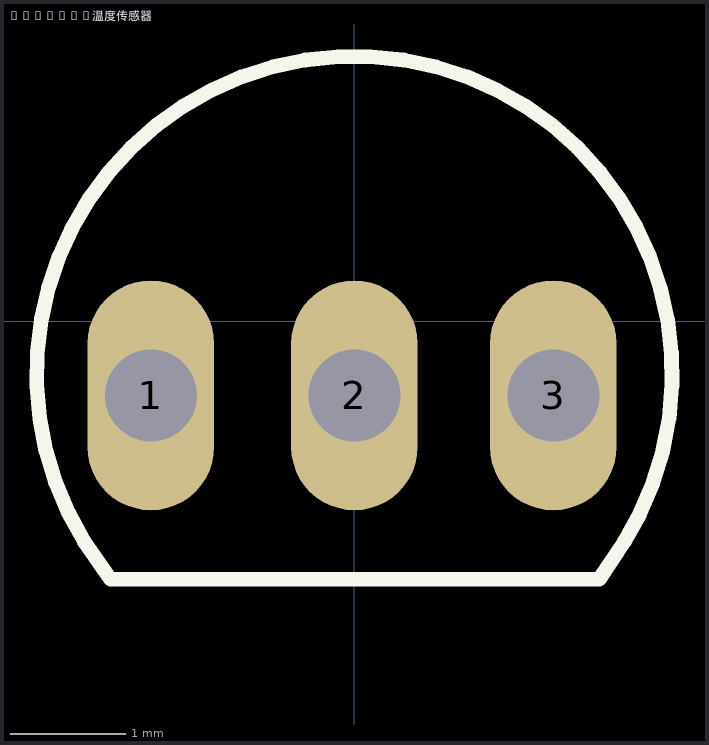
[diagram p0: the footprint, top view; thin cyan lines are the x and y axes]
# Altium footprint library MISC84237-10.PcbLib: 1 footprints
Each footprint in its own frame and in the unit in brackets; x right, y up, seen from the top. Pads: shape width x height; smd on the part's side, far side on the other; paste and mask are expansions set on the pad; w line width, h text height; cw(c..) or ccw(c..) is an arc to the next point about the centre after c.

## DS18B20温度传感器 [mm]
pads (3):
  oval 1.1x2 hole 0.8 paste+0 mask+0.051: 1(-1.77,-0.643) 2(0,-0.643) 3(1.73,-0.643)
Top Overlay:
  lines w0.127: -2.349,-1.914 cw(c0,-0.457) 2.349,-1.914 2.13,-2.243 -2.12,-2.243 -2.35,-1.913